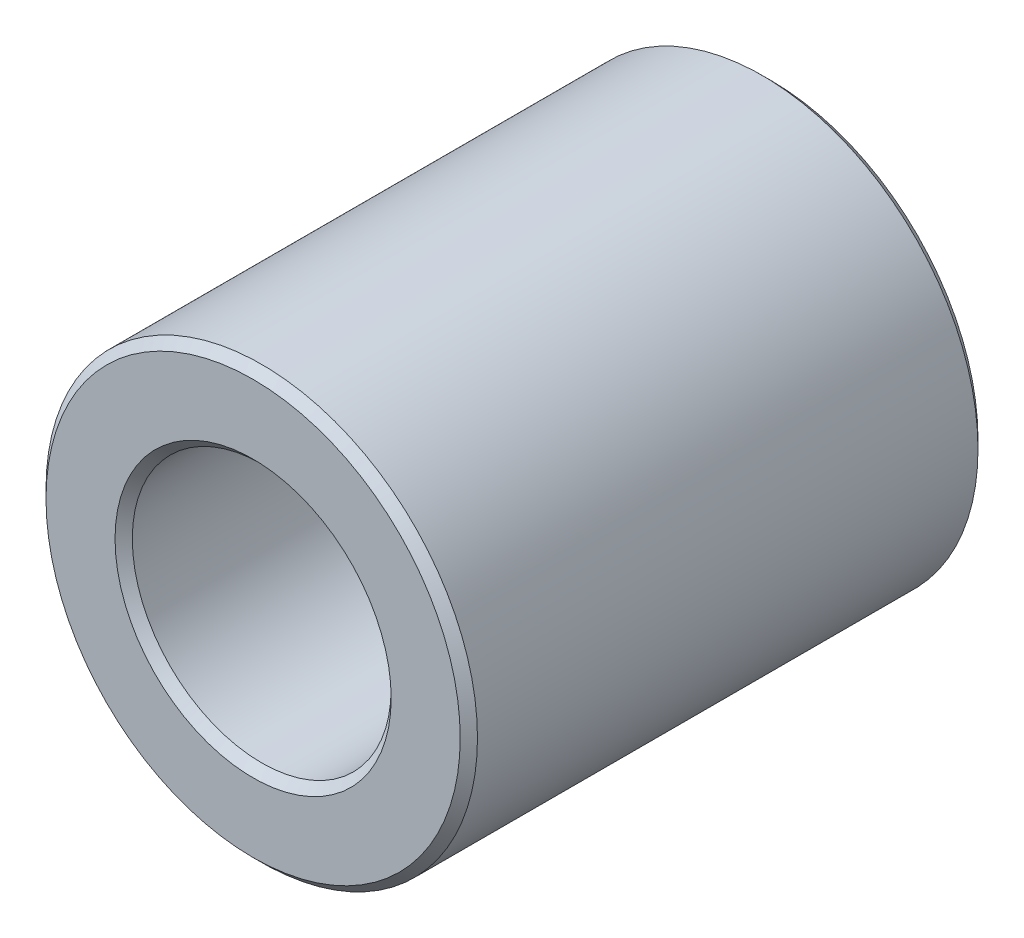
from build123d import *

# Parameters (mm, degrees)
SKETCH1_R           = 25
SKETCH1_R_2         = 15
BOSS_EXTRUDE1_DEPTH = 60
CHAMFER1_SIZE       = 1


with BuildPart() as part:
    # Sketch1 → Boss-Extrude1 (new body)
    with BuildSketch(Plane.XY):
        Circle(SKETCH1_R)
        Circle(SKETCH1_R_2, mode=Mode.SUBTRACT)
    extrude(amount=BOSS_EXTRUDE1_DEPTH)

    # Chamfer1
    chamfer1_edges = [part.edges().sort_by_distance(p)[0] for p in [
        (-25, 0, 0),
        (-25, 0, 60),
        (-15, 0, 0),
        (-15, 0, 60),
    ]]
    chamfer(chamfer1_edges, length=CHAMFER1_SIZE)


solid = part.part
